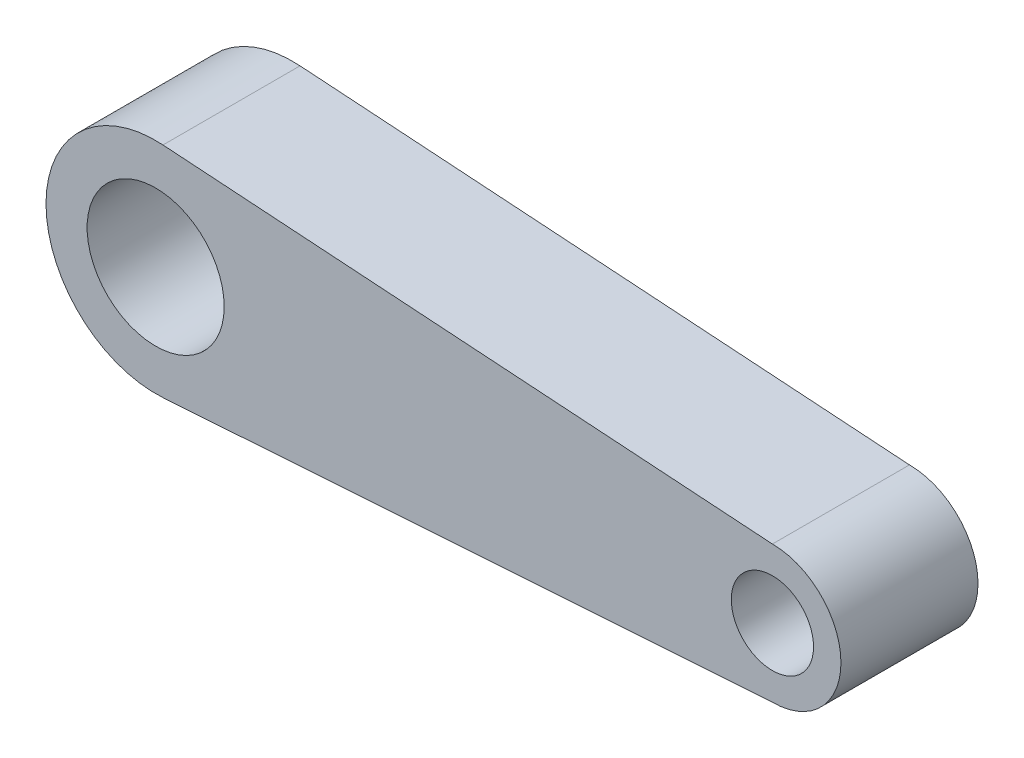
SolidWorks part; units mm, degrees
ref_plane "Front Plane" through (0, 0, 0) normal (0, 0, 1) x (1, 0, 0)
ref_plane "Top Plane" through (0, 0, 0) normal (0, 1, 0) x (1, 0, 0)
ref_plane "Right Plane" through (0, 0, 0) normal (1, 0, 0) x (0, 0, -1)
sketch "Sketch1" plane through (0, 0, 0) normal (0, 0, 1) x (1, 0, 0)
  line L0 (0, 0) -> (67.5, 0) construction
  line L1 (0.803, 11.9731) -> (67.5, 7.5)
  line L2 (0.803, -11.9731) -> (67.5, -7.5)
  circle A0 centre (0, 0) radius 7.5
  arc A1 (0.803, 11.9731) -> (0.803, -11.9731) centre (0, 0) ccw
  circle A2 centre (67.5, 0) radius 4.5
  arc A3 (67.5, -7.5) -> (67.5, 7.5) centre (67.5, 0) ccw
  dimension "D1" = 24
  dimension "D2" = 15
  dimension "D3" = 15
  dimension "D4" = 9
  dimension "D5" = 67.5
extrude "Boss-Extrude1" add sketch "Sketch1" along normal mid plane 15
